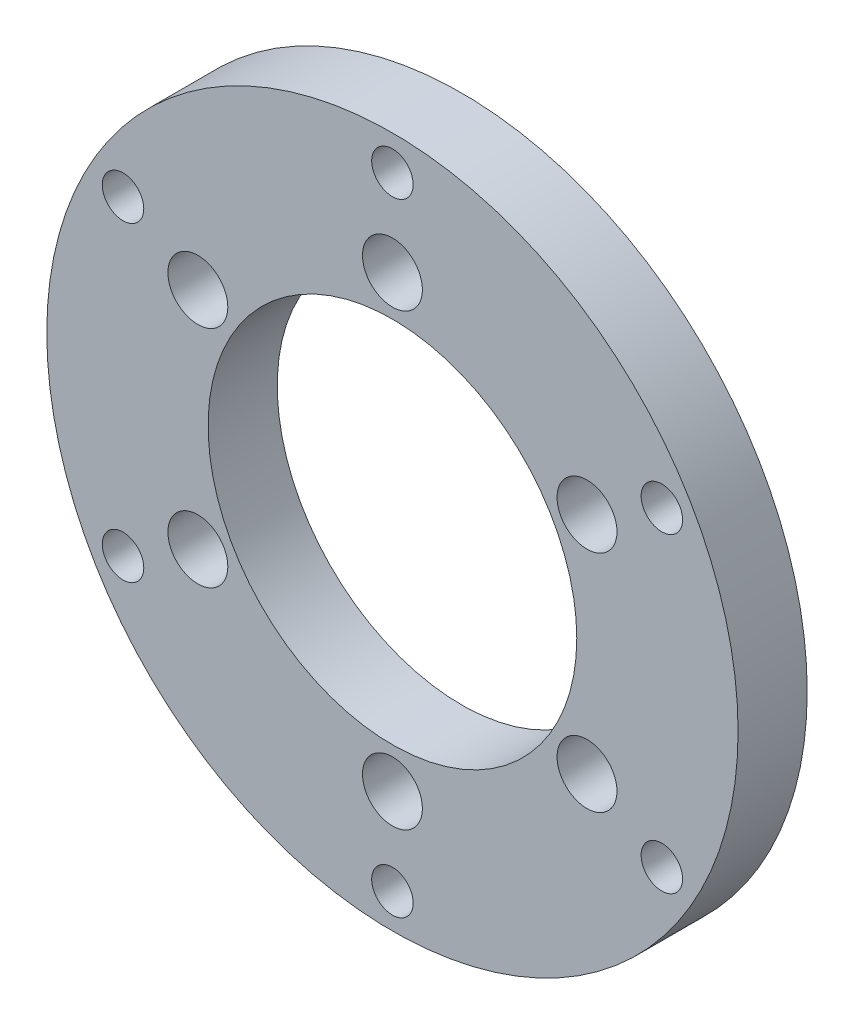
from build123d import *

# Parameters (mm, degrees)
SKETCH1_R           = 150
SKETCH1_R_2         = 80
BOSS_EXTRUDE1_DEPTH = 30
SKETCH2_R           = 9
CUT_EXTRUDE1_DEPTH  = 30
SKETCH3_R           = 9
CUT_EXTRUDE2_DEPTH  = 215.242852856
SKETCH4_R           = 13
CUT_EXTRUDE3_DEPTH  = 20


with BuildPart() as part:
    # Sketch1 → Boss-Extrude1 (new body)
    with BuildSketch(Plane.XY):
        Circle(SKETCH1_R)
        Circle(SKETCH1_R_2, mode=Mode.SUBTRACT)
    extrude(amount=BOSS_EXTRUDE1_DEPTH)

    # Sketch2 → Cut-Extrude1 (cut)
    with BuildSketch(Plane.XY.offset(30)):
        with Locations((0, 135)):
            Circle(SKETCH2_R)
        with Locations((116.913429511, 67.5)):
            Circle(SKETCH2_R)
        with Locations((116.913429511, -67.5)):
            Circle(SKETCH2_R)
        with Locations((0, -135)):
            Circle(SKETCH2_R)
        with Locations((-116.913429511, -67.5)):
            Circle(SKETCH2_R)
        with Locations((-116.913429511, 67.5)):
            Circle(SKETCH2_R)
    extrude(amount=-CUT_EXTRUDE1_DEPTH, mode=Mode.SUBTRACT)

    # Sketch3 → Cut-Extrude2 (cut, through all)
    with BuildSketch(Plane.XY.offset(30)):
        with Locations((0, 97.5)):
            Circle(SKETCH3_R)
        with Locations((84.437476869, 48.75)):
            Circle(SKETCH3_R)
        with Locations((84.437476869, -48.75)):
            Circle(SKETCH3_R)
        with Locations((0, -97.5)):
            Circle(SKETCH3_R)
        with Locations((-84.437476869, -48.75)):
            Circle(SKETCH3_R)
        with Locations((-84.437476869, 48.75)):
            Circle(SKETCH3_R)
    extrude(amount=-CUT_EXTRUDE2_DEPTH, mode=Mode.SUBTRACT)

    # Sketch4 → Cut-Extrude3 (cut)
    with BuildSketch(Plane.XY.offset(30)):
        with Locations((0, 97.5)):
            Circle(SKETCH4_R)
        with Locations((84.437476869, 48.75)):
            Circle(SKETCH4_R)
        with Locations((84.437476869, -48.75)):
            Circle(SKETCH4_R)
        with Locations((0, -97.5)):
            Circle(SKETCH4_R)
        with Locations((-84.437476869, -48.75)):
            Circle(SKETCH4_R)
        with Locations((-84.437476869, 48.75)):
            Circle(SKETCH4_R)
    extrude(amount=-CUT_EXTRUDE3_DEPTH, mode=Mode.SUBTRACT)


solid = part.part
